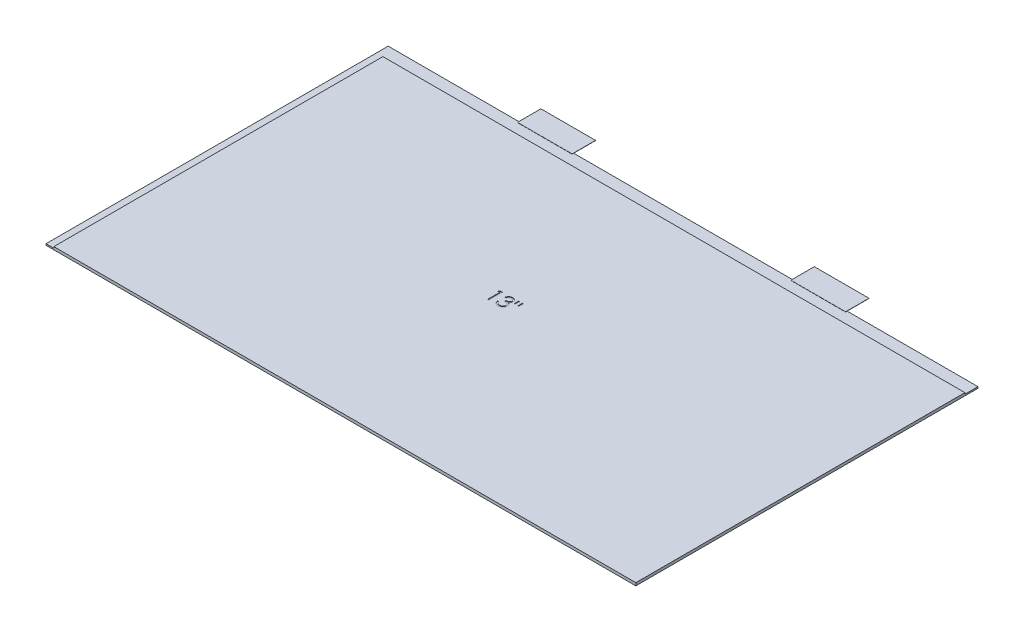
SolidWorks part; units mm, degrees
ref_plane "Front Plane" through (0, 0, 0) normal (0, 0, 1) x (1, 0, 0)
ref_plane "Top Plane" through (0, 0, 0) normal (0, 1, 0) x (1, 0, 0)
ref_plane "Right Plane" through (0, 0, 0) normal (1, 0, 0) x (0, 0, -1)
sketch "Sketch 2" plane through (0, 0, 0) normal (0, 1, 0) x (1, 0, 0)
  line L1 (-150.985, 87.595) -> (150.985, 87.595)
  line L2 (-150.985, 87.595) -> (-150.985, -87.595)
  line L3 (-150.985, -87.595) -> (150.985, -87.595)
  line L4 (150.985, 87.595) -> (150.985, -87.595)
  line L5 (-150.985, 87.595) -> (150.985, -87.595) construction
  line L6 (-150.985, -87.595) -> (150.985, 87.595) construction
  point P0 (0, 0)
  dimension "D1" = 301.97
  dimension "D2" = 175.19
extrude "Boss-Extrude 1" add sketch "Sketch 2" along normal blind 1.43
sketch "Sketch 4" plane through (0, 1.43, 0) normal (0, 1, 0) x (-1, 0, 0)
  line L0 (15, 0) -> (0, 0) construction
  text T0 "13\"" font "Century Gothic" height in points 20
  dimension "D1" = 15
extrude "Cut-Extrude 2" cut sketch "Sketch 4" against normal blind 0.2
sketch "Sketch 5" plane through (0, 1.43, 0) normal (0, 1, 0) x (1, 0, 0)
  line L1 (150.985, -87.595) -> (150.985, 87.595) construction
  line L2 (-150.985, 87.595) -> (150.985, 87.595)
  line L3 (-150.985, 87.595) -> (-150.985, 80.895)
  line L4 (-150.985, 80.895) -> (150.985, 80.895)
  line L5 (150.985, 87.595) -> (150.985, 80.895)
  dimension "D1" = 6.7
extrude "Cut-Extrude 3" cut sketch "Sketch 5" against normal blind 0.7
sketch "Sketch 6" plane through (0, 1.43, 0) normal (0, 1, 0) x (1, 0, 0)
  line L1 (-150.985, 80.895) -> (150.985, 80.895) construction
  line L2 (-150.985, -87.595) -> (-146.985, -87.595)
  line L3 (-150.985, -87.595) -> (-150.985, 80.895)
  line L4 (-150.985, 80.895) -> (-146.985, 80.895)
  line L5 (-146.985, -87.595) -> (-146.985, 80.895)
  dimension "D1" = 4
extrude "Cut-Extrude 4" cut sketch "Sketch 6" against normal up to surface (0.7 mm away) up to face at (0, 0.73, -84.245)
sketch "Sketch 7" plane through (0, 0.73, 0) normal (0, 1, 0) x (1, 0, 0)
  line L0 (150.985, 87.595) -> (-150.985, 87.595) construction
  line L1 (83.985, 86.795) -> (55.985, 86.795)
  line L2 (83.985, 86.795) -> (83.985, 98.795)
  line L3 (83.985, 98.795) -> (55.985, 98.795)
  line L4 (55.985, 86.795) -> (55.985, 98.795)
  line L5 (150.985, 80.895) -> (150.985, 87.595) construction
  point P6 (69.985, 86.795)
  dimension "D1" = 0.8
  dimension "D2" = 81
  dimension "D3" = 28
  dimension "D4" = 12
extrude "Boss-Extrude 2" add sketch "Sketch 7" along normal blind 0.1
pattern_linear "Linear Pattern 1" count 2 spacing 140 along (-1, 0, 0) of "Boss-Extrude 2"
